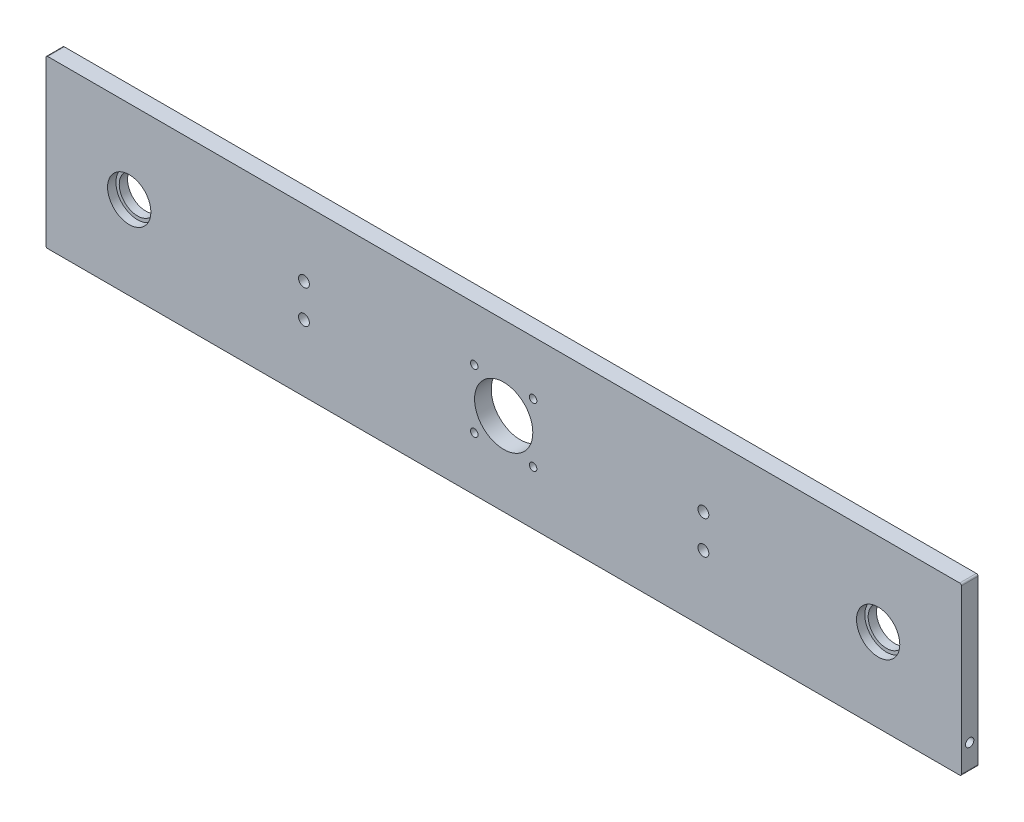
SolidWorks part; units mm, degrees
material "6061-T6 "
ref_plane "Front Plane" through (0, 0, 0) normal (0, 0, 1) x (1, 0, 0)
ref_plane "Top Plane" through (0, 0, 0) normal (0, 1, 0) x (1, 0, 0)
ref_plane "Right Plane" through (0, 0, 0) normal (1, 0, 0) x (0, 0, -1)
sketch "Sketch1" plane through (0, 0, 0) normal (0, 0, 1) x (1, 0, 0)
  line L1 (275, -50) -> (-275, -50)
  line L2 (275, -50) -> (275, 50)
  line L3 (275, 50) -> (-275, 50)
  line L4 (-275, -50) -> (-275, 50)
  line L5 (275, -50) -> (-275, 50) construction
  line L6 (275, 50) -> (-275, -50) construction
  point P0 (0, 0)
  dimension "D1" = 100
  dimension "D2" = 550
extrude "Boss-Extrude1" add sketch "Sketch1" along normal blind 10
sketch "Sketch3" plane through (0, 0, 10) normal (0, 0, 1) x (1, 0, 0)
  line L0 (0, 50) -> (0, -50) construction
  line L1 (275, 50) -> (-275, 50) construction
  line L2 (-275, -50) -> (275, -50) construction
  circle A0 centre (225, 0) radius 13
  circle A1 centre (-225, 0) radius 13
  dimension "D1" = 26
  dimension "D2" = 225
extrude "Cut-Extrude2" cut sketch "Sketch3" against normal blind 5
sketch "Sketch4" plane through (0, 0, 5) normal (0, 0, 1) x (1, 0, 0)
  line L0 (0, 50) -> (0, -50) construction
  line L1 (275, 50) -> (-275, 50) construction
  line L2 (-275, -50) -> (275, -50) construction
  circle A0 centre (225, 0) radius 11
  circle A1 centre (-225, 0) radius 11
  dimension "D1" = 22
extrude "Cut-Extrude3" cut sketch "Sketch4" against normal through all
sketch "Sketch5" plane through (0, 0, 10) normal (0, 0, 1) x (1, 0, 0)
  circle A0 centre (0, 0) radius 17.5
  dimension "D1" = 35
extrude "Cut-Extrude4" cut sketch "Sketch5" against normal through all
sketch "Sketch6" plane through (0, 0, 10) normal (0, 0, 1) x (1, 0, 0)
  line L0 (-17.6777, 17.6777) -> (17.6777, -17.6777) construction
  line L1 (-17.6777, -17.6777) -> (17.6777, 17.6777) construction
  line L2 (0, 0) -> (25, 0) construction
  circle A0 centre (0, 0) radius 25 construction
  circle A1 centre (-17.6777, 17.6777) radius 2.25
  circle A2 centre (17.6777, 17.6777) radius 2.25
  circle A3 centre (17.6777, -17.6777) radius 2.25
  circle A4 centre (-17.6777, -17.6777) radius 2.25
  dimension "D1" = 50
  dimension "D4" = 4.5
  dimension "D2" = 45
  dimension "D3" = 90
extrude "Cut-Extrude5" cut sketch "Sketch6" against normal through all
sketch "Sketch7" plane through (0, 0, 10) normal (0, 0, 1) x (1, 0, 0)
  line L0 (0, 50) -> (0, -50) construction
  line L1 (275, 50) -> (-275, 50) construction
  line L2 (-275, -50) -> (275, -50) construction
  line L3 (-275, 0) -> (275, 0) construction
  line L4 (-275, 50) -> (-275, -50) construction
  line L5 (275, -50) -> (275, 50) construction
  circle A2 centre (-120, -10) radius 3.25
  circle A3 centre (120, -10) radius 3.25
  circle A4 centre (120, 10) radius 3.25
  circle A5 centre (-120, 10) radius 3.25
  dimension "D2" = 20
  dimension "D1" = 240
  dimension "D3" = 6.5
extrude "Cut-Extrude6" cut sketch "Sketch7" against normal through all
fillet "Fillet1" radius 1 4 edges at (-275, -50, 5) (-275, 50, 5) (275, -50, 5) (275, 50, 5)
hole_wizard "M6 Tapped Hole1" positions "Sketch8" profile "Sketch9" tap size "M6" standard "GB"
sketch "Sketch8" plane through (-275, 0, 0) normal (-1, 0, 0) x (0, 0, 1)
  line L0 (10, 49) -> (0, 49) construction
  line L1 (10, -50) -> (0, -50) construction
  point P0 (5, -35)
  point P7 (5, 49)
  dimension "D1" = 15
sketch "Sketch9" plane through (-275, -35, 5) normal (0, 1, 0) x (0, 0, 1)
  line L0 (0, 0) -> (0, 19.5022)
  line L1 (0, 19.5022) -> (2.5, 18)
  line L2 (2.5, 18) -> (2.5, 0)
  line L5 (2.5, 0) -> (0, 0)
  line L10 (0, 19.5022) -> (-2.5, 18) construction
  line L11 (0, -6.35) -> (0, 107.95) construction
  dimension "螺纹孔钻头直径" = 5
  dimension "螺纹孔钻头深度" = 18
  dimension "导头角度" = 118
cosmetic thread "Hole Thread1" parameters "D1"=15, "D2"=6
mirror "Mirror1" about plane through (0, 0, 0) normal (1, 0, 0) of "M6 Tapped Hole1"
